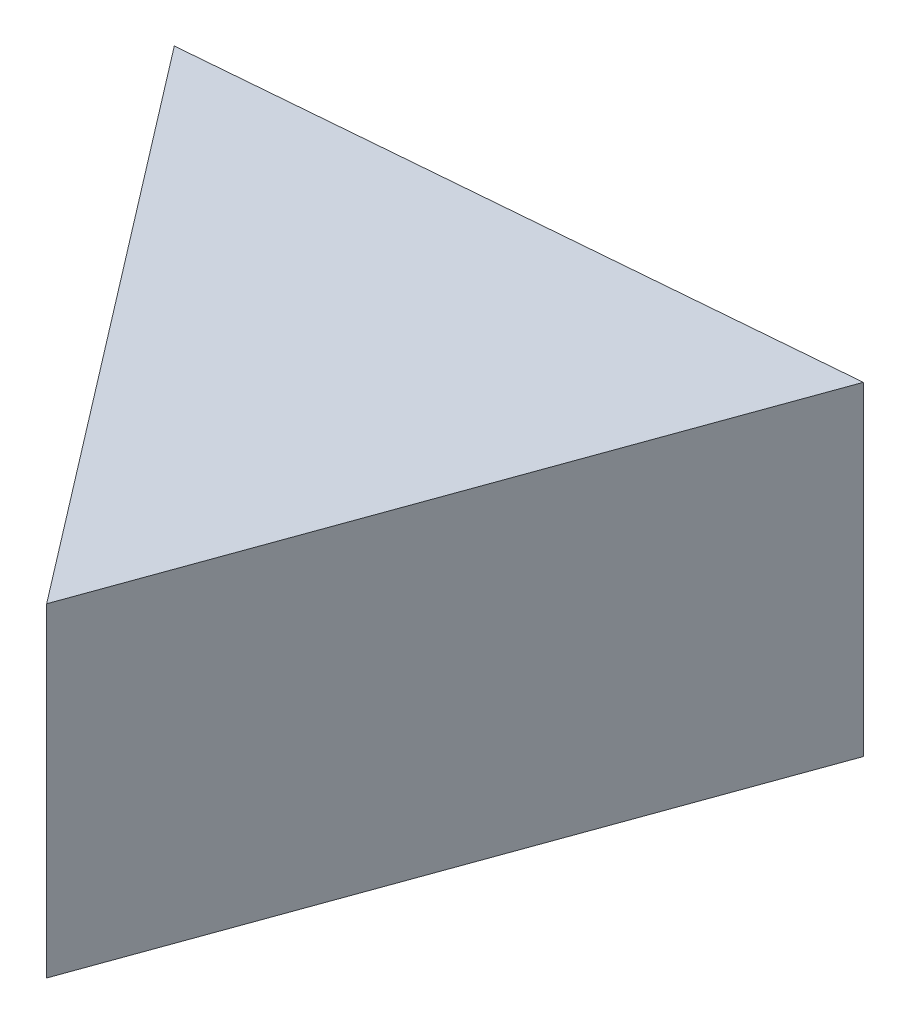
from build123d import *

# Parameters (mm, degrees)
BOSS_EXTRUDE1_DEPTH = 12.7


with BuildPart() as part:
    # Sketch1 → Boss-Extrude1 (new body)
    with BuildSketch(Plane(origin=(0, 0, 0), x_dir=(1, 0, 0), z_dir=(0, 1, 0))):
        Polygon((0, 0), (-24.912712211, -2.087287789), (-8.486277569, -23.515592551), align=None)
    extrude(amount=BOSS_EXTRUDE1_DEPTH)


solid = part.part
